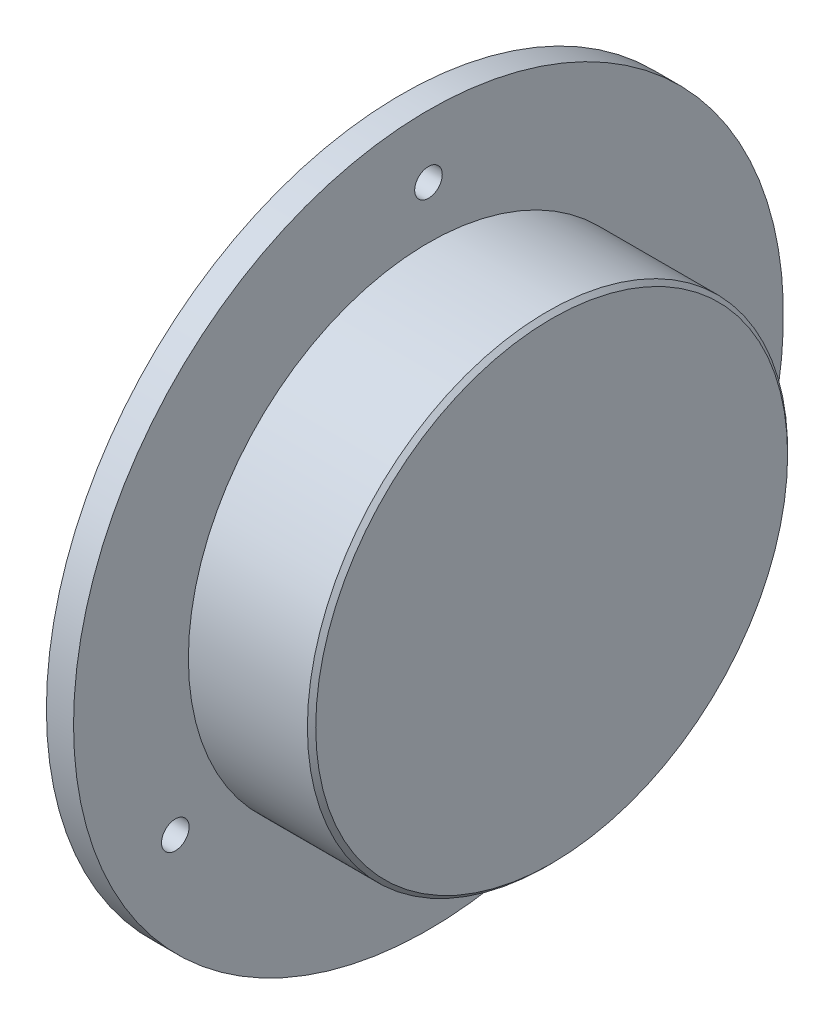
from build123d import *

# Parameters (mm, degrees)
HOLE_WIZARD_M6_1_D = 6.6
CHAMFER_1_SIZE     = 1


with BuildPart() as part:
    # 草图2 → 旋转1 (revolve)
    with BuildSketch(Plane.XY, mode=Mode.PRIVATE) as revolve_1_sk:
        Polygon((30, 0), (30, 50), (0, 50), (0, 85), (6.5, 85), (6.5, 57.5), (36, 57.5), (36, 0), align=None)
    revolve(revolve_1_sk.sketch.rotate(Axis((0, 0, 0), (1, 0, 0)), 90), axis=Axis((0, 0, 0), (1, 0, 0)))

    # M6 间隙孔1 (through all)
    with Locations(Plane(origin=(6.5, 0, 0), x_dir=(0, 0, -1), z_dir=(1, 0, 0))):
        with Locations((-60.621778265, -35), (0, 70), (60.621778265, -35)):
            Hole(HOLE_WIZARD_M6_1_D / 2)

    # 倒角1
    chamfer_1_edges = [part.edges().sort_by_distance(p)[0] for p in [
        (36, 0, -57.5),
    ]]
    chamfer(chamfer_1_edges, length=CHAMFER_1_SIZE)


solid = part.part
